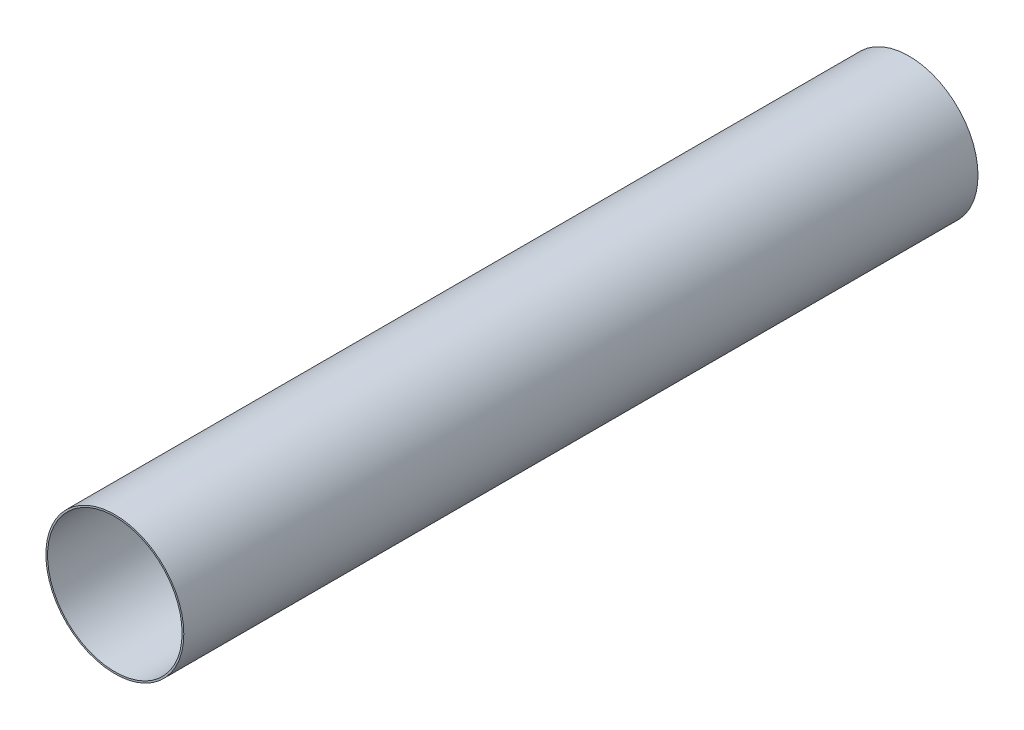
from build123d import *

# Parameters (mm, degrees)
SKETCH_1_R      = 48.5
SKETCH_1_R_2    = 47.3
EXTRUDE_1_DEPTH = 558.5


with BuildPart() as part:
    # 草图1 → 凸台-拉伸1 (new body)
    with BuildSketch(Plane.XY):
        Circle(SKETCH_1_R)
        Circle(SKETCH_1_R_2, mode=Mode.SUBTRACT)
    extrude(amount=EXTRUDE_1_DEPTH)


solid = part.part
